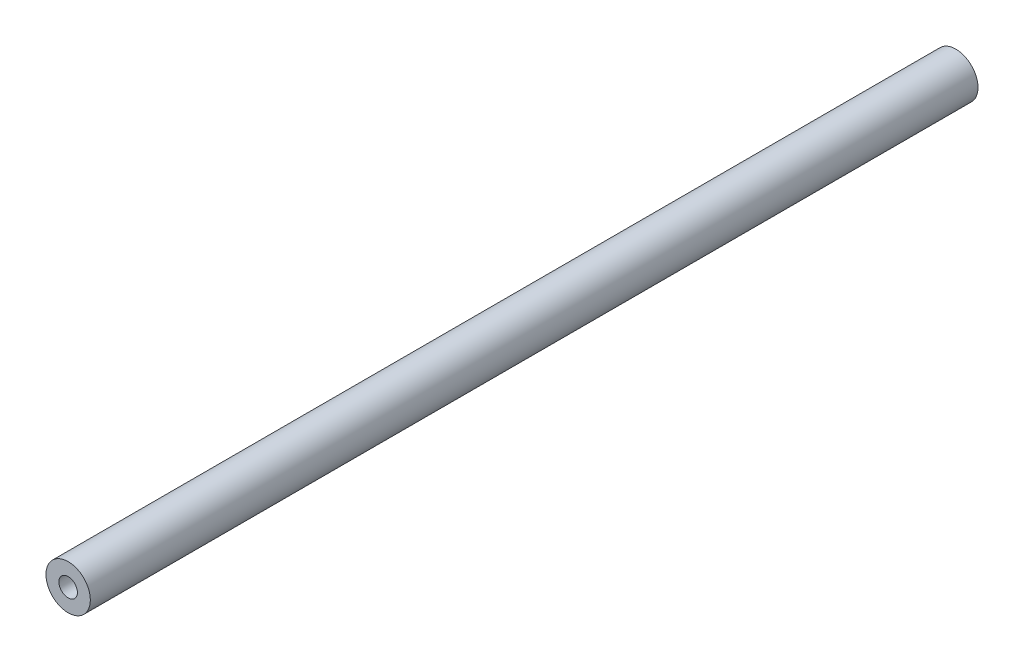
from build123d import *

# Parameters (mm, degrees)
SKETCH1_R             = 3
BOSS_EXTRUDE1_DEPTH   = 120
M3_TAPPED_HOLE1_D     = 2.5
M3_TAPPED_HOLE1_DEPTH = 8.5
M3_TAPPED_HOLE1_TIP   = 0.751075774
M3_TAPPED_HOLE2_D     = 2.5
M3_TAPPED_HOLE2_DEPTH = 8.5
M3_TAPPED_HOLE2_TIP   = 0.751075774


with BuildPart() as part:
    # Sketch1 → Boss-Extrude1 (new body)
    with BuildSketch(Plane.XY):
        Circle(SKETCH1_R)
    extrude(amount=BOSS_EXTRUDE1_DEPTH)

    # M3 Tapped Hole1
    with Locations(Plane.XY.offset(120)):
        with Locations((0, 0)):
            Hole(M3_TAPPED_HOLE1_D / 2, depth=M3_TAPPED_HOLE1_DEPTH)
            with Locations((0, 0, -(M3_TAPPED_HOLE1_DEPTH + M3_TAPPED_HOLE1_TIP / 2))):  # 118° drill point
                Cone(0, M3_TAPPED_HOLE1_D / 2, M3_TAPPED_HOLE1_TIP, mode=Mode.SUBTRACT)

    # M3 Tapped Hole2
    with Locations(Plane(origin=(0, 0, 0), x_dir=(-1, 0, 0), z_dir=(0, 0, -1))):
        with Locations((0, 0)):
            Hole(M3_TAPPED_HOLE2_D / 2, depth=M3_TAPPED_HOLE2_DEPTH)
            with Locations((0, 0, -(M3_TAPPED_HOLE2_DEPTH + M3_TAPPED_HOLE2_TIP / 2))):  # 118° drill point
                Cone(0, M3_TAPPED_HOLE2_D / 2, M3_TAPPED_HOLE2_TIP, mode=Mode.SUBTRACT)


solid = part.part
